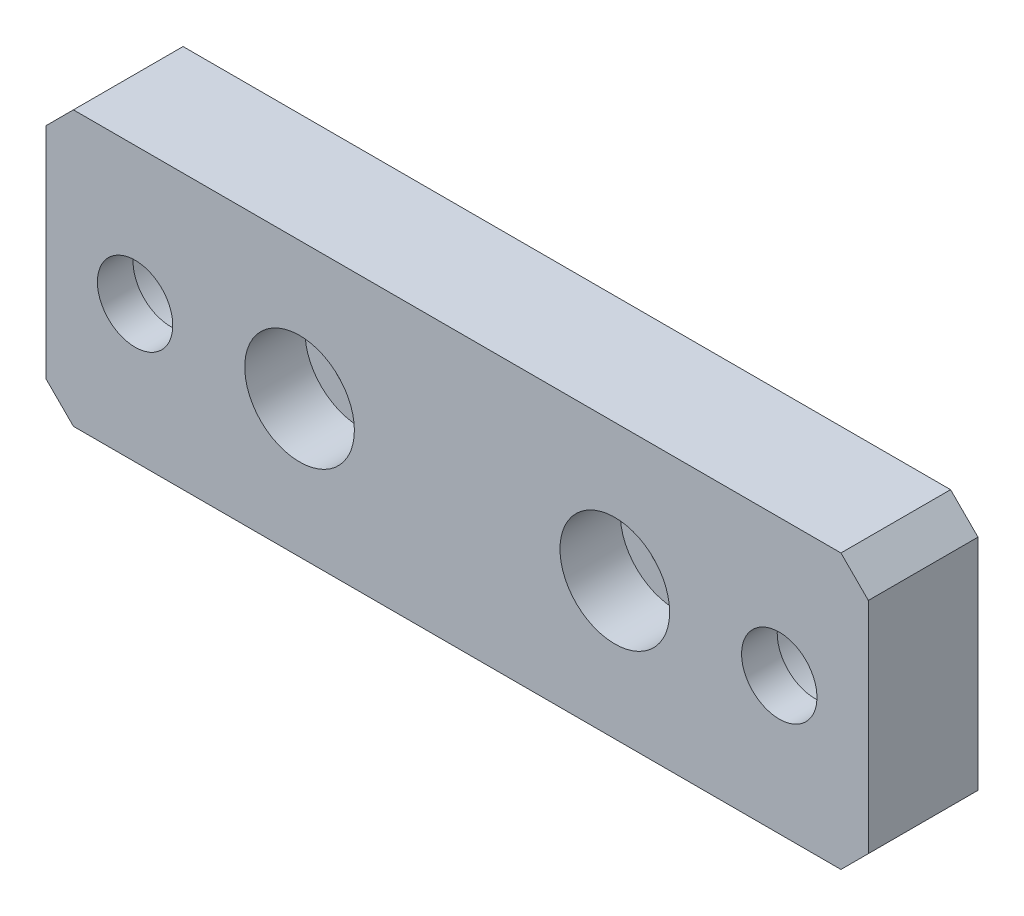
SolidWorks part; units mm, degrees
material "AL6061"
ref_plane "Front" through (0, 0, 0) normal (0, 0, 1) x (1, 0, 0)
ref_plane "Top" through (0, 0, 0) normal (0, 1, 0) x (1, 0, 0)
ref_plane "Right" through (0, 0, 0) normal (1, 0, 0) x (0, 0, -1)
sketch "Sketch1" plane through (0, 0, 0) normal (0, 0, 1) x (1, 0, 0)
  line L1 (0, 0) -> (60, 0)
  line L2 (0, 0) -> (0, 20)
  line L3 (0, 20) -> (60, 20)
  line L4 (60, 0) -> (60, 20)
  dimension "D1" = 20
  dimension "D2" = 60
extrude "Boss-Extrude1" add sketch "Sketch1" along normal blind 8
hole_wizard "CBORE for M4 Hex Socket Head Cap Screw2" positions "Sketch2" profile "Sketch3" counterbore size "M4" standard "ISO" end condition through all
sketch "Sketch2" plane through (0, 0, 8) normal (0, 0, 1) x (1, 0, 0)
  line L0 (30, 20) -> (30, 0) construction
  line L1 (60, 20) -> (0, 20) construction
  line L2 (0, 0) -> (60, 0) construction
  line L5 (0, 10) -> (60, 10) construction
  line L6 (0, 20) -> (0, 0) construction
  line L7 (60, 0) -> (60, 20) construction
  point P18 (18.5, 10)
  point P23 (41.5, 10)
  dimension "D1" = 23
  dimension "D2" = 10
sketch "Sketch3" plane through (41.5, 10, 8) normal (1, 0, 0) x (0, -1, 0)
  line L0 (0, 0) -> (0, 8)
  line L1 (0, 8) -> (2.25, 8)
  line L3 (2.25, 8) -> (2.25, 4.4)
  line L4 (2.25, 4.4) -> (4, 4.4)
  line L5 (4, 4.4) -> (4, 0)
  line L7 (4, 0) -> (0, 0)
  line L11 (0, -6.35) -> (0, 107.95) construction
  dimension "通孔孔直径" = 4.5
  dimension "通孔孔深度" = 8
  dimension "柱形沉头孔直径" = 8
  dimension "柱形沉头孔深度" = 4.4
hole_wizard "CBORE for M5 Hex Socket Head Cap Screw1" positions "Sketch4" profile "Sketch5" counterbore size "M5" standard "ISO" end condition through all
sketch "Sketch4" plane through (0, 0, 0) normal (0, 0, 1) x (1, 0, 0)
  line L0 (0, 10) -> (60, 10) construction
  line L1 (0, 20) -> (0, 0) construction
  line L2 (60, 0) -> (60, 20) construction
  line L5 (30, 20) -> (30, 0) construction
  line L6 (60, 20) -> (0, 20) construction
  line L7 (0, 0) -> (60, 0) construction
  point P19 (6.5, 10)
  point P22 (53.5, 10)
  dimension "D1" = 6.5
sketch "Sketch5" plane through (53.5, 10, 0) normal (1, 0, 0) x (0, 1, 0)
  line L0 (0, 0) -> (0, 8)
  line L1 (0, 8) -> (2.75, 8)
  line L3 (2.75, 8) -> (2.75, 5.4)
  line L4 (2.75, 5.4) -> (5, 5.4)
  line L5 (5, 5.4) -> (5, 0)
  line L7 (5, 0) -> (0, 0)
  line L11 (0, -6.35) -> (0, 107.95) construction
  dimension "通孔孔直径" = 5.5
  dimension "通孔孔深度" = 8
  dimension "柱形沉头孔直径" = 10
  dimension "柱形沉头孔深度" = 5.4
chamfer "Chamfer1" distance 2 angle 45 4 edges at (60, 20, 4) (60, 0, 4) (0, 20, 4) (0, 0, 4)
